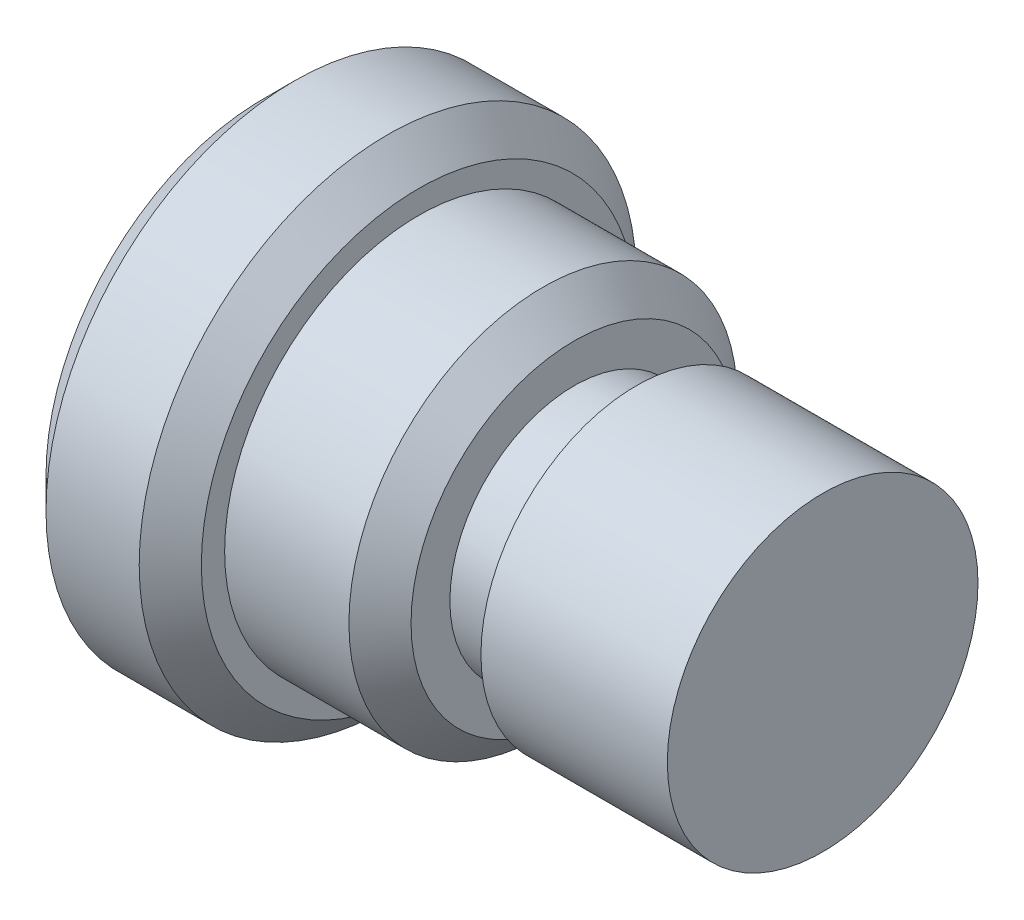
SolidWorks part; units mm, degrees
material "45#"
ref_plane "前视基准面" through (0, 0, 0) normal (0, 0, 1) x (1, 0, 0)
ref_plane "上视基准面" through (0, 0, 0) normal (0, 1, 0) x (1, 0, 0)
ref_plane "右视基准面" through (0, 0, 0) normal (1, 0, 0) x (0, 0, -1)
sketch "草图1" plane through (0, 0, 0) normal (0, 0, 1) x (1, 0, 0)
  line L0 (-129.4448, -89.1184) -> (-104.4448, -89.1184) construction
  line L1 (-129.4448, -112.1184) -> (-129.4448, -79.1184) construction
  line L2 (-123.4448, -82.8684) -> (-129.4448, -82.8684) construction
  line L4 (-116.4448, -84.1184) -> (-122.4448, -84.1184)
  line L5 (-122.4448, -84.1184) -> (-122.4448, -85.1184)
  line L6 (-122.4448, -85.1184) -> (-124.4448, -85.1184)
  line L7 (-124.4448, -85.1184) -> (-124.4448, -82.8684)
  line L8 (-124.4448, -82.8684) -> (-129.4448, -82.8684)
  line L9 (-129.4448, -82.8684) -> (-129.4448, -81.1184)
  line L10 (-129.4448, -81.1184) -> (-134.4448, -81.1184)
  line L11 (-134.4448, -81.1184) -> (-134.4448, -89.1184)
  line L12 (-116.4448, -84.1184) -> (-116.4448, -89.1184)
  line L16 (-134.4448, -89.1184) -> (-116.4448, -89.1184)
  point P18 (0, 0)
  point P20 (0, 0)
  point P21 (0, 0)
  dimension "D1" = 6.25
  dimension "D2" = 12.5
  dimension "D3" = 16
  dimension "D4" = 5
  dimension "D5" = 5
  dimension "D6" = 2
  dimension "D7" = 1
  dimension "D8" = 10
  dimension "D9" = 6
revolve "旋转1" add sketch "草图1" angle 360 about L0
cosmetic thread "装饰螺纹线1" parameters "D2"=8.376
chamfer "倒角1" distance 1 angle 45 3 edges at (-134.4448, -89.1184, 8) (-129.4448, -89.1184, 8) (-124.4448, -89.1184, 6.25)
